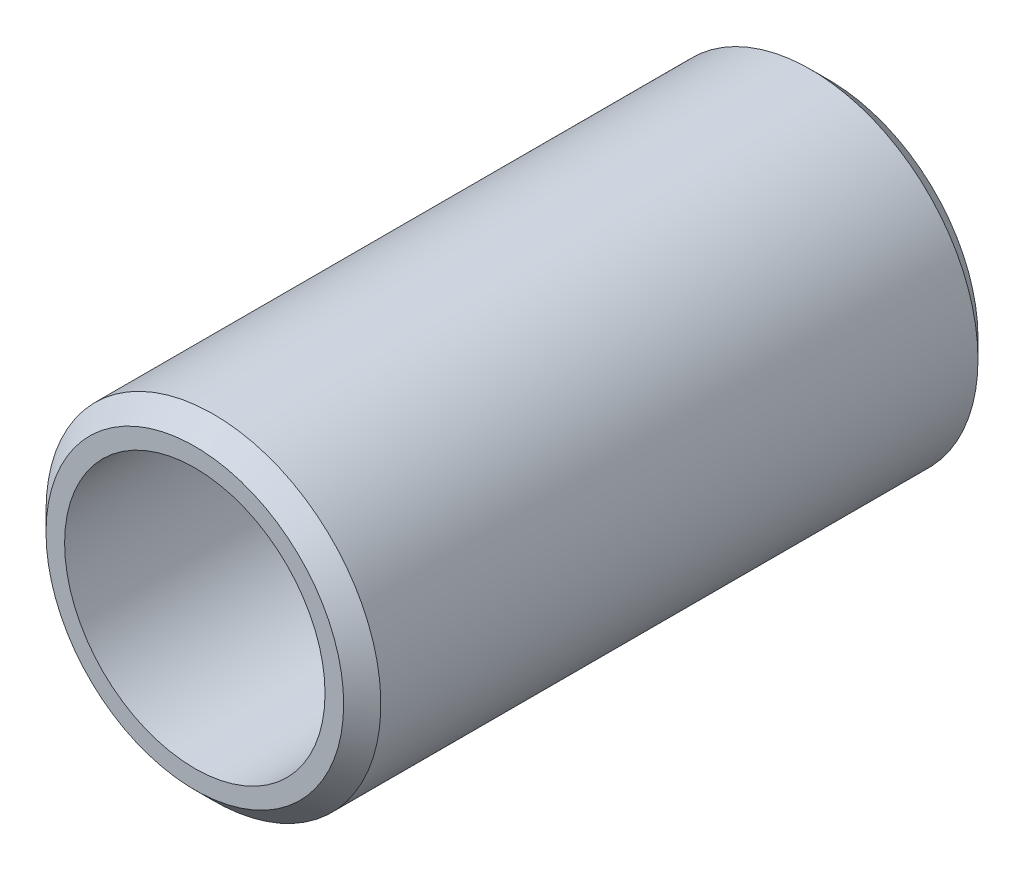
SolidWorks part; units mm, degrees
ref_plane "Front Plane" through (0, 0, 0) normal (0, 0, 1) x (1, 0, 0)
ref_plane "Top Plane" through (0, 0, 0) normal (0, 1, 0) x (1, 0, 0)
ref_plane "Right Plane" through (0, 0, 0) normal (1, 0, 0) x (0, 0, -1)
sketch "Sketch2" plane through (0, 0, 0) normal (0, 0, 1) x (1, 0, 0)
  circle A0 centre (0, 0) radius 90
  circle A1 centre (0, 0) radius 70
  dimension "D1" = 180
  dimension "D2" = 140
extrude "Boss-Extrude1" add sketch "Sketch2" along normal blind 341
chamfer "Chamfer1" distance 10 angle 45 2 edges at (90, 0, 0) (90, 0, 341)
